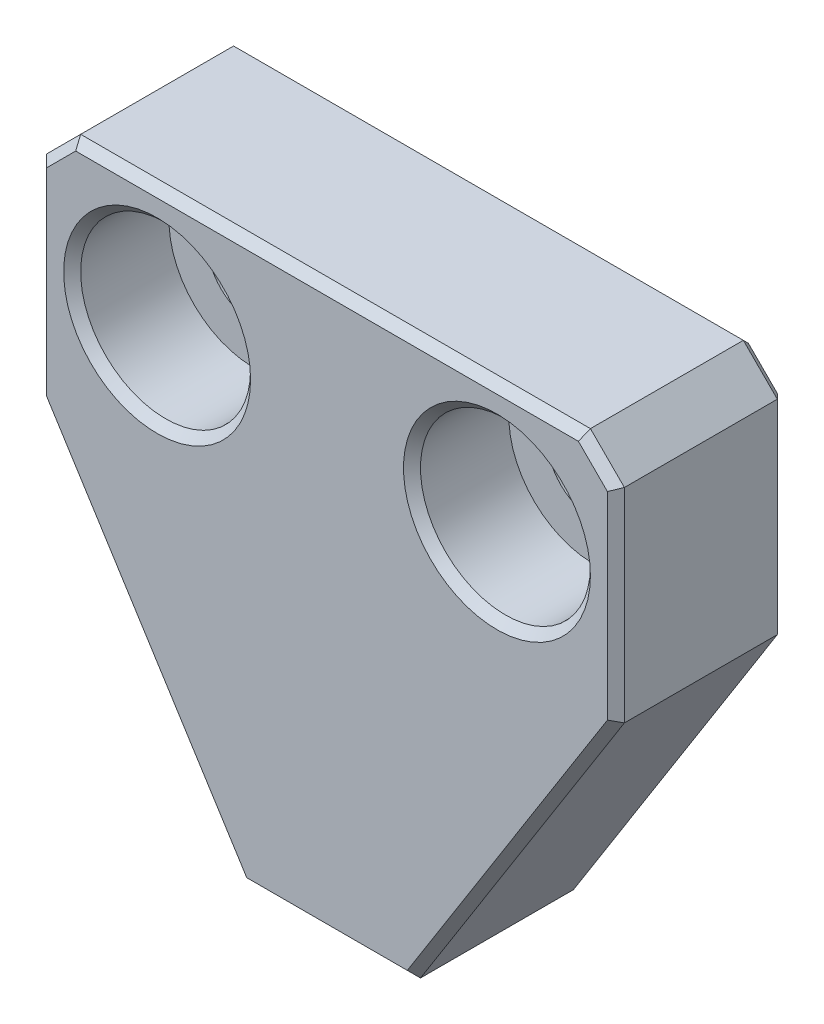
SolidWorks part; units mm, degrees
material "Aluminum Profile"
ref_plane "Front Plane" through (0, 0, 0) normal (0, 0, 1) x (1, 0, 0)
ref_plane "Top Plane" through (0, 0, 0) normal (0, 1, 0) x (1, 0, 0)
ref_plane "Right Plane" through (0, 0, 0) normal (1, 0, 0) x (0, 0, -1)
sketch "Sketch1" plane through (0, 0, 0) normal (0, 0, 1) x (1, 0, 0)
  line L1 (17, -7) -> (-17, -7)
  line L2 (17, -7) -> (17, 7)
  line L3 (17, 7) -> (-17, 7)
  line L4 (-17, -7) -> (-17, 7)
  line L5 (17, -7) -> (-17, 7) construction
  line L6 (17, 7) -> (-17, -7) construction
  point P0 (0, 0)
  dimension "D1" = 34
  dimension "D2" = 14
extrude "Boss-Extrude1" add sketch "Sketch1" along normal blind 10
hole_wizard "Hole size per socket head cap screw type1" positions "3DSketch1" profile "Sketch2" counterbore size "M5" standard "Gb" end condition through all
sketch3d "3DSketch1"
  line L0 (-10, 0, 10) -> (10, 0, 10) construction
  line L2 (0, 7, 10) -> (0, 0, 10) construction
  line L3 (17, 7, 10) -> (-17, 7, 10) construction
  point P0 (-10, 0, 10)
  point P2 (10, 0, 10)
  dimension "D1" = 7
  dimension "D2" = 20
sketch "Sketch2" plane through (-10, 0, 10) normal (1, 0, 0) x (0, -1, 0)
  line L0 (0, 0) -> (0, 10)
  line L1 (0, 10) -> (2.75, 10)
  line L3 (2.75, 10) -> (2.75, 5.7)
  line L4 (2.75, 5.7) -> (5, 5.7)
  line L5 (5, 5.7) -> (5, 0)
  line L7 (5, 0) -> (0, 0)
  line L11 (0, -6.35) -> (0, 107.95) construction
  dimension "通孔孔直径" = 5.5
  dimension "通孔孔深度" = 10
  dimension "柱形沉头孔直径" = 10
  dimension "柱形沉头孔深度" = 5.7
sketch "Sketch3" plane through (0, 0, 10) normal (0, 0, 1) x (1, 0, 0)
  line L0 (-17, -7) -> (-5, -26)
  line L1 (-5, -26) -> (5, -26)
  line L2 (5, -26) -> (17, -7)
  line L3 (17, -7) -> (-17, -7)
  dimension "D1" = 10
  dimension "D2" = 19
extrude "Boss-Extrude2" add sketch "Sketch3" against normal up to surface (10 mm away) up to face at (-7.25, 0, 0)
chamfer "Chamfer2" distance 2 angle 45 2 edges at (-17, 7, 5) (17, 7, 5)
chamfer "Chamfer1" distance 0.5 angle 45 20 edges at (0, 7, 10) (17, -1, 10) (-17, -1, 10) (15, 0, 10) (-5, 0, 10) (11, -16.5, 0) (11, -16.5, 10) (0, -26, 0) (0, -26, 10) (-11, -16.5, 0) (-11, -16.5, 10) (17, -1, 0) (0, 7, 0) (-17, -1, 0) (12.75, 0, 0) (-7.25, 0, 0) (16, 6, 0) (-16, 6, 0) (16, 6, 10) (-16, 6, 10)
